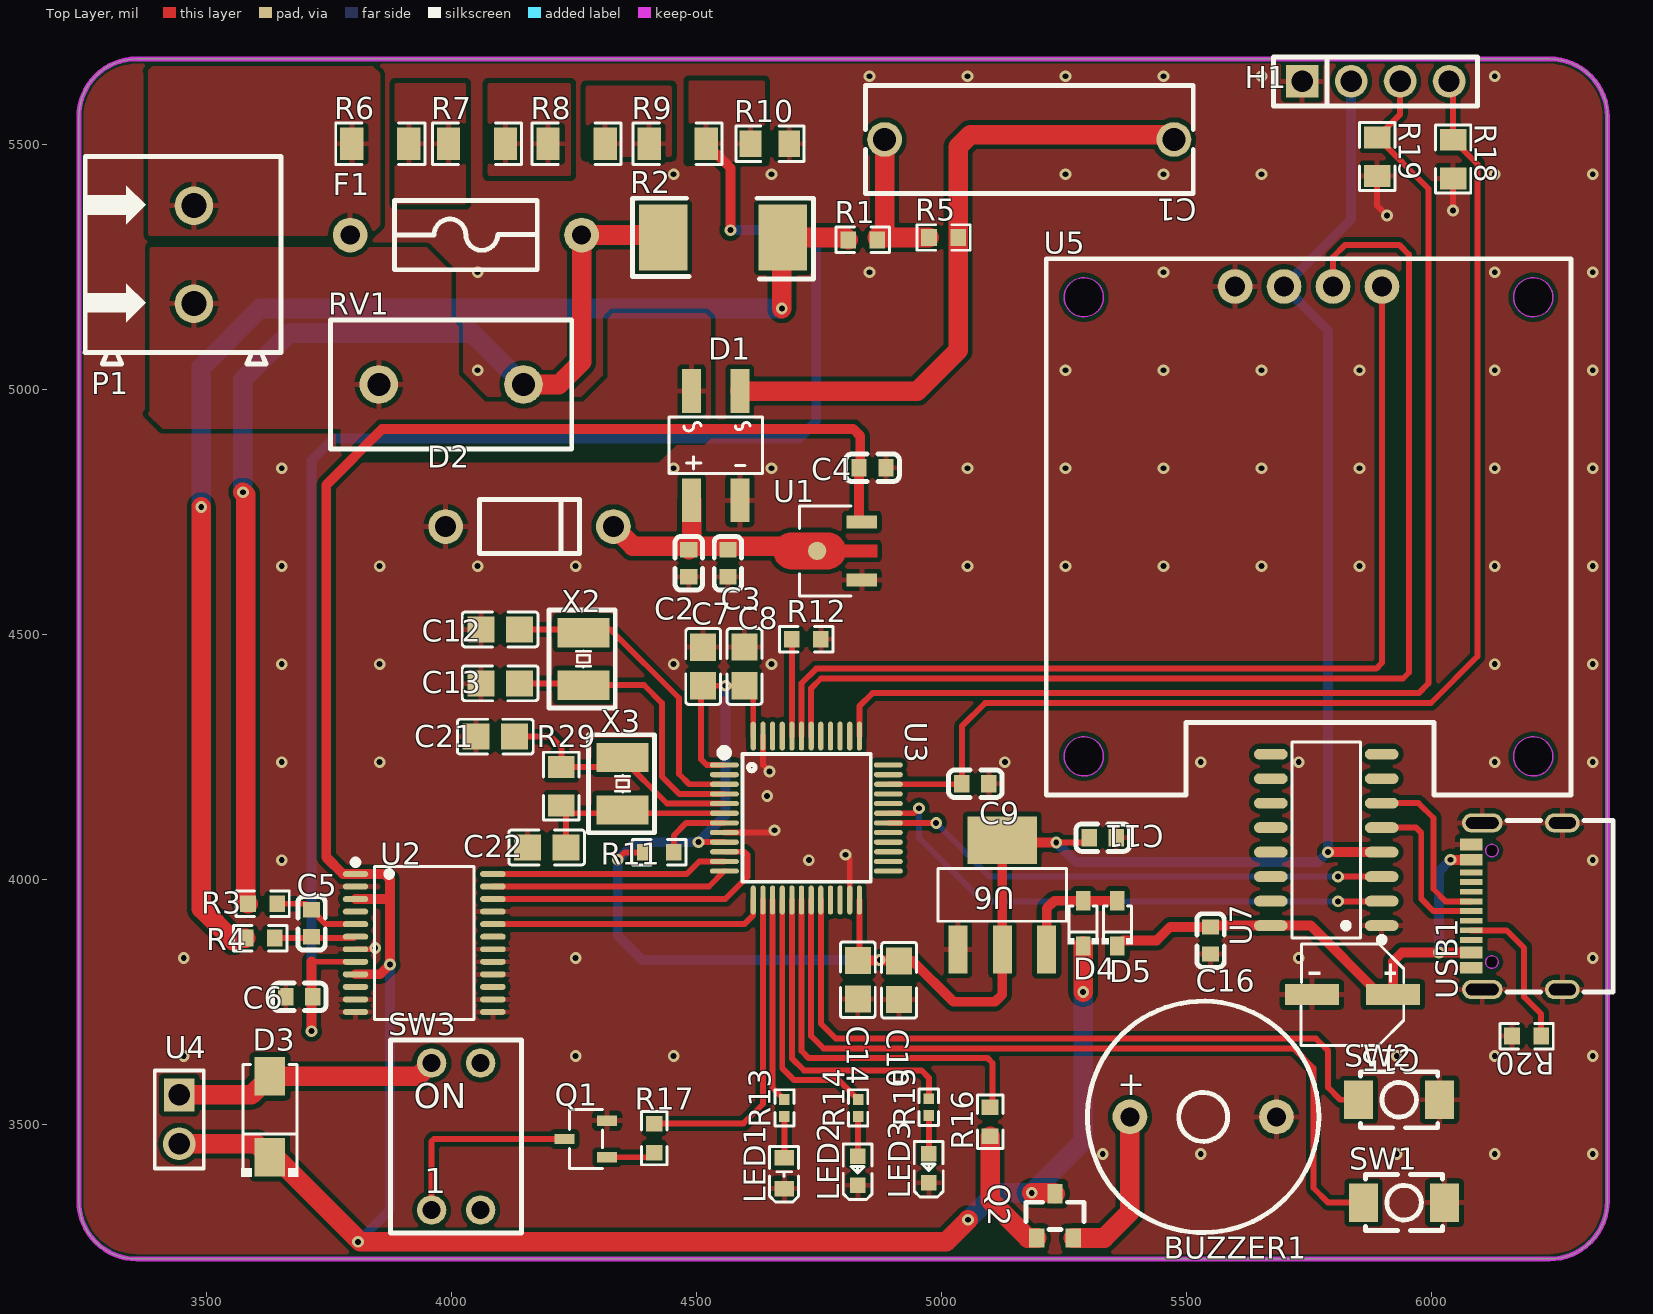
[diagram p0: Top Layer view]
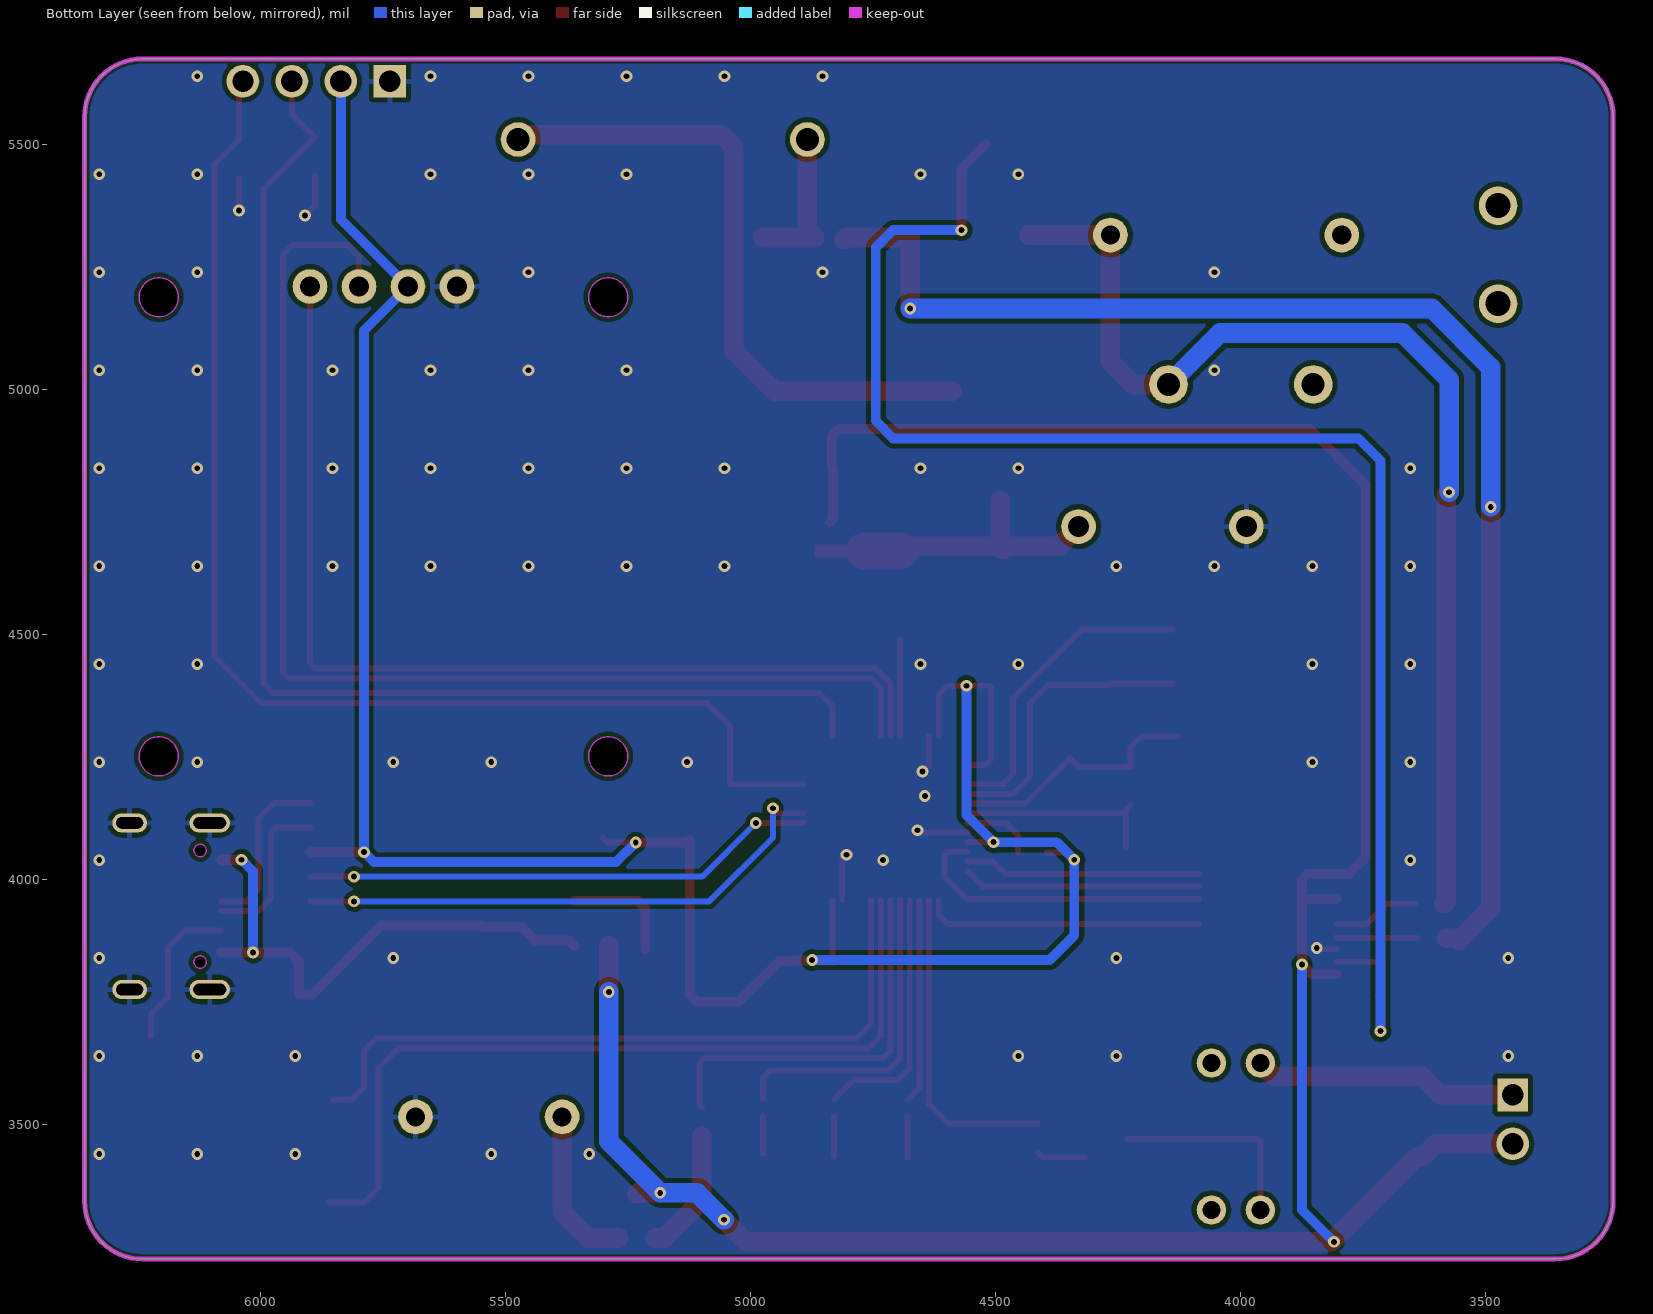
[diagram p1: Bottom Layer view, seen from below]
# Altium PCB MISC49877.pcbdoc
Units mil, origin at the board's own origin, x right, y up, seen from the top; angles counter-clockwise.
Board outline 3120 x 2449.61 mil, 2 copper layers (Top Layer, Bottom Layer), stack 2.757 mil thick; 67 components, 52 nets, 243 pads, 106 vias.

## Layer stack, top to bottom
Top Solder Mask Layer: solder mask 0.394, Dk 3.3
Top Layer: signal copper 1.379
Bottom Layer: signal copper 1.378
Bottom Solder Mask Layer: solder mask 0.394, Dk 3.3

## Board outline
3358.11,5674.61 ccw(c3358.11,5556.5) 3240,5556.5 3240,3343.11 ccw(c3358.11,3343.11) 3358.11,3225 6241.89,3225 ccw(c6241.89,3343.11) 6360,3343.11 6360,5556.5 ccw(c6241.89,5556.5) 6241.89,5674.61 3358.11,5674.61

## Design rules (kind name [scope] priority, off if disabled: settings)
BoardOutlineClearance Plane_innerPlane_1 [All] p2 off: genericclearance=4 ignorepadtopadclearanceinfootprint=FALSE except(0: Arc-SplitContinuation Track-SplitContinuation SMDPad-SplitContinuation THPad-SplitContinuation Via-SplitContinuation Fill-SplitContinuation Region-SplitContinuation Poly-SplitContinuation Text-SplitContinuation Hole-SplitContinuation; 6: Arc-CutoutEdge Track-CutoutEdge SMDPad-CutoutEdge THPad-CutoutEdge Via-CutoutEdge Text-CutoutEdge; 6.9: Hole-OutlineEdge Hole-CutoutEdge; 10: Poly-OutlineEdge Poly-CutoutEdge; 11.8: Arc-OutlineEdge Track-OutlineEdge SMDPad-OutlineEdge THPad-OutlineEdge Via-OutlineEdge Fill-OutlineEdge Region-OutlineEdge Text-OutlineEdge Fill-CutoutEdge Region-CutoutEdge)
BoardOutlineClearance Copper_copperRegion_1 [All] p4 off: genericclearance=4 ignorepadtopadclearanceinfootprint=FALSE except(0: Arc-SplitContinuation Track-SplitContinuation SMDPad-SplitContinuation THPad-SplitContinuation Via-SplitContinuation Fill-SplitContinuation Region-SplitContinuation Poly-SplitContinuation Text-SplitContinuation Hole-SplitContinuation; 6: Arc-CutoutEdge Track-CutoutEdge SMDPad-CutoutEdge THPad-CutoutEdge Via-CutoutEdge Text-CutoutEdge; 6.9: Hole-OutlineEdge Hole-CutoutEdge; 10: Poly-OutlineEdge Poly-CutoutEdge; 11.8: Arc-OutlineEdge Track-OutlineEdge SMDPad-OutlineEdge THPad-OutlineEdge Via-OutlineEdge Fill-OutlineEdge Region-OutlineEdge Text-OutlineEdge Fill-CutoutEdge Region-CutoutEdge)
BoardOutlineClearance Copper_copperRegion_copperThickness1oz_1 [All] p6 off: genericclearance=4 ignorepadtopadclearanceinfootprint=FALSE except(0: Arc-SplitContinuation Track-SplitContinuation SMDPad-SplitContinuation THPad-SplitContinuation Via-SplitContinuation Fill-SplitContinuation Region-SplitContinuation Poly-SplitContinuation Text-SplitContinuation Hole-SplitContinuation; 6: Arc-CutoutEdge Track-CutoutEdge SMDPad-CutoutEdge THPad-CutoutEdge Via-CutoutEdge Text-CutoutEdge; 6.9: Hole-OutlineEdge Hole-CutoutEdge; 10: Poly-OutlineEdge Poly-CutoutEdge; 11.8: Arc-OutlineEdge Track-OutlineEdge SMDPad-OutlineEdge THPad-OutlineEdge Via-OutlineEdge Fill-OutlineEdge Region-OutlineEdge Text-OutlineEdge Fill-CutoutEdge Region-CutoutEdge)
BoardOutlineClearance Copper_copperRegion_Copper_copperRegion_1 [All] p8 off: genericclearance=4 ignorepadtopadclearanceinfootprint=FALSE except(0: Arc-SplitContinuation Track-SplitContinuation SMDPad-SplitContinuation THPad-SplitContinuation Via-SplitContinuation Fill-SplitContinuation Region-SplitContinuation Poly-SplitContinuation Text-SplitContinuation Hole-SplitContinuation; 6: Arc-CutoutEdge Track-CutoutEdge SMDPad-CutoutEdge THPad-CutoutEdge Via-CutoutEdge Text-CutoutEdge; 6.9: Hole-OutlineEdge Hole-CutoutEdge; 10: Poly-OutlineEdge Poly-CutoutEdge; 11.8: Arc-OutlineEdge Track-OutlineEdge SMDPad-OutlineEdge THPad-OutlineEdge Via-OutlineEdge Fill-OutlineEdge Region-OutlineEdge Text-OutlineEdge Fill-CutoutEdge Region-CutoutEdge)
BoardOutlineClearance copperThickness1oz_1 [All] p10: genericclearance=4 ignorepadtopadclearanceinfootprint=FALSE except(0: Arc-SplitContinuation Track-SplitContinuation SMDPad-SplitContinuation THPad-SplitContinuation Via-SplitContinuation Fill-SplitContinuation Region-SplitContinuation Poly-SplitContinuation Text-SplitContinuation Hole-SplitContinuation; 6: Arc-CutoutEdge Track-CutoutEdge SMDPad-CutoutEdge THPad-CutoutEdge Via-CutoutEdge Text-CutoutEdge; 6.9: Hole-OutlineEdge Hole-CutoutEdge; 10: Poly-OutlineEdge Poly-CutoutEdge; 11.8: Arc-OutlineEdge Track-OutlineEdge SMDPad-OutlineEdge THPad-OutlineEdge Via-OutlineEdge Fill-OutlineEdge Region-OutlineEdge Text-OutlineEdge Fill-CutoutEdge Region-CutoutEdge)
Clearance Plane_innerPlane [All] p1 off: gap=4 ignorepadtopadclearanceinfootprint=FALSE except(6: SMDPad-Track SMDPad-SMDPad THPad-Track SMDPad-THPad THPad-THPad Track-Via SMDPad-Via THPad-Via Via-Via Fill-SMDPad Region-SMDPad Fill-THPad Region-THPad Fill-Via Region-Via Fill-Fill Fill-Region Region-Region Arc-Track Arc-SMDPad Arc-THPad Arc-Via Fill-Arc Region-Arc Arc-Arc Text-Track SMDPad-Text Text-THPad Text-Via Fill-Text Region-Text Arc-Text Text-Text; 6.9: Hole-Track Hole-SMDPad Hole-THPad Hole-Via Fill-Hole Region-Hole Hole-Arc Hole-Text; 10: Poly-Track Poly-SMDPad Poly-THPad Poly-Via Poly-Fill Poly-Region Poly-Poly Poly-Arc Poly-Text Poly-Hole; 11.8: Fill-Track Region-Track)
Clearance Copper_copperRegion [All] p3 off: gap=4 ignorepadtopadclearanceinfootprint=FALSE except(6: SMDPad-Track SMDPad-SMDPad THPad-Track SMDPad-THPad THPad-THPad Track-Via SMDPad-Via THPad-Via Via-Via Fill-SMDPad Region-SMDPad Fill-THPad Region-THPad Fill-Via Region-Via Fill-Fill Fill-Region Region-Region Arc-Track Arc-SMDPad Arc-THPad Arc-Via Fill-Arc Region-Arc Arc-Arc Text-Track SMDPad-Text Text-THPad Text-Via Fill-Text Region-Text Arc-Text Text-Text; 6.9: Hole-Track Hole-SMDPad Hole-THPad Hole-Via Fill-Hole Region-Hole Hole-Arc Hole-Text; 10: Poly-Track Poly-SMDPad Poly-THPad Poly-Via Poly-Fill Poly-Region Poly-Poly Poly-Arc Poly-Text Poly-Hole; 11.8: Fill-Track Region-Track)
Clearance Copper_copperRegion_copperThickness1oz [All] p5 off: gap=4 ignorepadtopadclearanceinfootprint=FALSE except(6: SMDPad-Track SMDPad-SMDPad THPad-Track SMDPad-THPad THPad-THPad Track-Via SMDPad-Via THPad-Via Via-Via Fill-SMDPad Region-SMDPad Fill-THPad Region-THPad Fill-Via Region-Via Fill-Fill Fill-Region Region-Region Arc-Track Arc-SMDPad Arc-THPad Arc-Via Fill-Arc Region-Arc Arc-Arc Text-Track SMDPad-Text Text-THPad Text-Via Fill-Text Region-Text Arc-Text Text-Text; 6.9: Hole-Track Hole-SMDPad Hole-THPad Hole-Via Fill-Hole Region-Hole Hole-Arc Hole-Text; 10: Poly-Track Poly-SMDPad Poly-THPad Poly-Via Poly-Fill Poly-Region Poly-Poly Poly-Arc Poly-Text Poly-Hole; 11.8: Fill-Track Region-Track)
Clearance Copper_copperRegion_Copper_copperRegion [All] p7 off: gap=4 ignorepadtopadclearanceinfootprint=FALSE except(6: SMDPad-Track SMDPad-SMDPad THPad-Track SMDPad-THPad THPad-THPad Track-Via SMDPad-Via THPad-Via Via-Via Fill-SMDPad Region-SMDPad Fill-THPad Region-THPad Fill-Via Region-Via Fill-Fill Fill-Region Region-Region Arc-Track Arc-SMDPad Arc-THPad Arc-Via Fill-Arc Region-Arc Arc-Arc Text-Track SMDPad-Text Text-THPad Text-Via Fill-Text Region-Text Arc-Text Text-Text; 6.9: Hole-Track Hole-SMDPad Hole-THPad Hole-Via Fill-Hole Region-Hole Hole-Arc Hole-Text; 10: Poly-Track Poly-SMDPad Poly-THPad Poly-Via Poly-Fill Poly-Region Poly-Poly Poly-Arc Poly-Text Poly-Hole; 11.8: Fill-Track Region-Track)
Clearance copperThickness1oz [All] p9: gap=4 ignorepadtopadclearanceinfootprint=FALSE except(6: SMDPad-Track SMDPad-SMDPad THPad-Track SMDPad-THPad THPad-THPad Track-Via SMDPad-Via THPad-Via Via-Via Fill-SMDPad Region-SMDPad Fill-THPad Region-THPad Fill-Via Region-Via Fill-Fill Fill-Region Region-Region Arc-Track Arc-SMDPad Arc-THPad Arc-Via Fill-Arc Region-Arc Arc-Arc Text-Track SMDPad-Text Text-THPad Text-Via Fill-Text Region-Text Arc-Text Text-Text; 6.9: Hole-Track Hole-SMDPad Hole-THPad Hole-Via Fill-Hole Region-Hole Hole-Arc Hole-Text; 10: Poly-Track Poly-SMDPad Poly-THPad Poly-Via Poly-Fill Poly-Region Poly-Poly Poly-Arc Poly-Text Poly-Hole; 11.8: Fill-Track Region-Track)
DiffPairsRouting differentialPair [All] p1: maxlimit=6 minlimit=5 mostfreqgap=6 toplayer_minwidth=5 toplayer_prefwidth=100 toplayer_maxwidth=100 toplayer_mingap=5 toplayer_prefgap=6 toplayer_maxgap=6 bottomlayer_minwidth=5 bottomlayer_prefwidth=100 bottomlayer_maxwidth=100 bottomlayer_mingap=5 bottomlayer_prefgap=6 bottomlayer_maxgap=6 maxuncoupledlength=10
HoleToHoleClearance otherClearance [All] p1: gap=11.8 allowstackedmicrovias=TRUE
Length netLength [All] p1: minlimit=0 maxlimit=0
MatchedLengths netLengthTolerance [All] p1: tolerance=1000
PasteMaskExpansion pasteMaskExpansion [All] p1: expansion=0
PlaneConnect innerPlane [All] p1: planeconnectstyle=Relief reliefexpansion=20 reliefentries=4 reliefconductorwidth=10 reliefairgap=10
PolygonConnect copperRegion_copperThickness1oz [All] p1 off: connectstyle=Relief reliefconductorwidth=10 reliefentries=4 polygonreliefangle="90 Angle" airgapwidth=10 via.connectstyle=Relief via.reliefconductorwidth=10 via.reliefentries=4 via.polygonreliefangle="90 Angle" via.airgapwidth=10
PolygonConnect copperRegion_Copper_copperRegion [All] p2 off: connectstyle=Relief reliefconductorwidth=10 reliefentries=4 polygonreliefangle="90 Angle" airgapwidth=10 via.connectstyle=Relief via.reliefconductorwidth=10 via.reliefentries=4 via.polygonreliefangle="90 Angle" via.airgapwidth=10
PolygonConnect copperRegion [All] p3: connectstyle=Direct reliefconductorwidth=10 reliefentries=4 polygonreliefangle="90 Angle" airgapwidth=10 via.connectstyle=Relief via.reliefconductorwidth=10 via.reliefentries=4 via.polygonreliefangle="90 Angle" via.airgapwidth=10
RoutingVias viaSize [All] p1: holewidth=12 width=24 viastyle="Through Hole" minholewidth=1 minwidth=1 maxholewidth=393.7 maxwidth=248
SolderMaskExpansion solderMaskExpansion [IsVia] p1: expansion=-1000 istentingtop=TRUE
SolderMaskExpansion solderMaskExpansion [All] p2: expansion=2 istentingtop=FALSE
Width copperThickness1oz_2 [All] p1: maxlimit=100 minlimit=5 preferedwidth=10

## Components (designator, comment, footprint, x,y, rotation, side; value= is the part's Value field where it differs from the comment)
BUZZER1 "2.4kHz" BUZ-TH_BD12.0-P7.60-D0.6-FD 5535,3515 r0 top
C1 "470nF" CAP-TH_L17.0-W5.5-P15.00-D1.2 5180,5510 r180 top
C2 "100μF" C0603 4485,4645 r90 top
C3 "0.1μF" C0603 4565,4645 r270 top
C4 "10μF" C0603 4860,4840 r180 top
C5 "1nF" C0603 3715,3910 r90 top
C6 "1nF" C0603 3690,3760 r0 top
C7 "100nF" C0805 4514.37,4434.37 r90 top
C8 "100nF" C0805 4598.8,4434.51 r270 top
C9 "100nF" C0603 5070,4195 r180 top
C10 "100nF" C0805 4914.37,3793.97 r270 top
C11 "100nF" C0603 5330,4085 r180 top
C12 "20pF" C0805 4100,4510 r180 top
C13 "20pF" C0805 4100,4400 r0 top
C14 "100nF" C0805 4830,3795 r90 top
C15 "10uF" CAP-SMD_BD5.0-L5.3-W5.3-FD 5839.64,3765 r180 top
C16 "100nF" C0603 5550,3875 r90 top
C21 "20pF" C0805 4090.21,4291.12 r0 top
C22 "20pF" C0805 4195,4065 r0 top
D1 "MB10S" MBS_L4.7-W4.0-P2.50-LS7.0-TL 4540,4885 r270 top
D2 "1N4742" DO-41_BD2.4-L4.7-P8.70-D0.8-FD 4160,4720 r0 top
D3 "1N4007" SMA_L4.3-W2.5-LS5.0-RD 3630,3515 r90 top
D4 "1N5819WS" SOD-323_L1.8-W1.3-LS2.5-RD 5290,3910 r90 top
D5 "1N5819WS" SOD-323_L1.8-W1.3-LS2.5-RD 5360,3910 r90 top
F1 "2F.0500212000S1B02" FUSE-TH_BD3.0-L7.2-P11.20-D0.6 4030,5315 r0 top
H1 "" HDR-TH_4P-P2.54-V-F 5887,5628.78 r0 top
LED1 "NCD0603G1" LED0603-RD_1 4679.87,3400.05 r90 top
LED2 "NCD0603R1" LED0603-RD_RED 4830,3405 r90 top
LED3 "NCD0603Y1" LED0603-RD 4975,3410 r90 top
P1 "WJ500V-5.08-2P" CONN-TH_2P-P5.00_WJ500V-5.08-2P 3475,5275 r90 top
Q1 "S8050 J3Y(RANGE:200-350)" SOT-23-3_L3.0-W1.7-P0.95-LS2.9-BR 4275,3470 r0 top
Q2 "" S8050_SOT-23 5232.54,3313.14 r270 top
R1 "10Ω" R0603 4840,5305 r0 top
R2 "2mΩ" RES-SMD_L6.4-W3.2-1 4555,5310 r0 top
R3 "1K" R0603 3615,3950 r0 top
R4 "1K" R0603 3610,3880 r0 top
R5 "1MΩ" R0603 5005,5310 r0 top
R6 "1MΩ" R1206 3855.45,5501.36 r0 top
R7 "1MΩ" R1206 4052.86,5501.36 r0 top
R8 "1MΩ" R1206 4256.06,5501.36 r0 top
R9 "1MΩ" R1206 4462.27,5501.36 r0 top
R10 "10kΩ" R0805 4650.66,5501.36 r0 top
R11 "10K" R0603 4425,4055 r0 top
R12 "10K" R0603 4725,4490 r0 top
R13 "220Ω" R0402 4680.3,3533.26 r90 top
R14 "220Ω" R0402 4830.69,3533.26 r90 top
R15 "220Ω" R0402 4975,3535 r90 top
R16 "1KΩ" R0603 5100,3505 r90 top
R17 "1KΩ" R0603 4414.48,3471.81 r270 top
R18 "10kΩ" R0805 6045,5470 r270 top
R19 "10kΩ" R0805 5890,5475 r270 top
R20 "5.1K" R0603 6195,3680 r180 top
R29 "1M" R0805 4225,4190 r90 top
RV1 "190pF@1kHz" RES-TH_L12.5-W6.7-P7.50-D1.2 4000,5010 r0 top
SW1 "TS3425A2P 250gf" SW-SMD_L3.9-W2.9-LS5.0 5945,3340 r0 top
SW2 "TS3425A2P 250gf" SW-SMD_L3.9-W2.9-LS5.0 5935,3550 r0 top
SW3 "BSE02GR" SW-TH_4P-L9.9-W6.8-P7.62-BL 4010,3475 r0 top
U1 "HT7550-1" SOT-89_L4.5-W2.5-P1.50-LS4.2-BR 4785,4670 r0 top
U2 "ADE7755ARSZ" SSOP-24_L8.1-W5.3-P0.65-LS7.8-BL 3945,3870 r270 top
U3 "STM32F030C8T6TR" LQFP-48_L7.0-W7.0-P0.50-LS9.0-BL 4725,4125 r270 top
U4 "KF301-5.0-2P" HDR-M-2.54_1X2 3445,3510 r270 top
U5 "HS96L03W2C03" OLED-TH_L27.8-W27.2-P2.54_C9900033791 5750,5210 r0 top
U6 "AMS1117-3.3" SOT-223-4_L6.5-W3.5-P2.30-LS7.0-BR 5125,3968.34 r270 top
U7 "CH340C" SOP-16_L10.0-W3.9-P1.27-LS6.0-BL 5786.23,4080.41 r90 top
USB1 "TYPE-C16PIN" USB-C-SMD_TYPE-C16PIN 6175,3945 r90 top
X2 "32.768MHz" CRYSTAL-SMD_L3.2-W2.5_3225-8MHZ 4270,4450 r90 top
X3 "8MHz" CRYSTAL-SMD_L3.2-W2.5_3225-8MHZ 4350,4195 r90 top

## Footprints (in the part's own frame and the unit in brackets; to place one, negate y for a bottom-side part, rotate by r counter-clockwise, add the part's x,y. Pads: shape width x height; smd on the part's side, far side on the other; paste and mask are expansions set on the pad)
BUZ-TH_BD12.0-P7.60-D0.6-FD [mm]
  round 1.8 hole 1: 1(-3.8,0) 2(3.8,0)
  silkscreen extent -6,-6 6,6
C0603 [mm]
  rect 0.8x0.9 smd: 1(-0.7,0) 2(0.7,0)
  silkscreen extent -1.39,-0.71 1.39,0.71
C0805 [mm]
  rect 1.41x1.35 smd paste-100 mask+0.051: 1(-1,0) 2(1,0)
  silkscreen extent -1.96,-0.9 1.96,0.9
CAP-SMD_BD5.0-L5.3-W5.3-FD [mm]
  rect 2.8x1.1 smd: 1(-2.1,0) 2(2.1,0)
  silkscreen extent -2.66,-2.62 2.66,2.65
CAP-TH_L17.0-W5.5-P15.00-D1.2 [mm]
  round 1.8 hole 1.2: 1(-7.501,0) 2(7.501,0)
  silkscreen extent -8.5,-2.8 8.5,2.8
CONN-TH_2P-P5.00_WJ500V-5.08-2P [mm]
  round 2 hole 1.3: 1(-2.54,0) 2(2.54,0)
  silkscreen extent -5.68,-4.52 5.08,5.64
CRYSTAL-SMD_L3.2-W2.5_3225-8MHZ [mil]
  rect 60x106.3 smd paste+0 mask+1.97: 1(-53.62,0) 2(53.62,0)
  silkscreen extent -100,-65 100,70
DO-41_BD2.4-L4.7-P8.70-D0.8-FD [mm]
  round 1.8 hole 1.1: 1(-4.35,0) 2(4.35,0)
  silkscreen extent -2.6,-1.4 2.6,1.4
FUSE-TH_BD3.0-L7.2-P11.20-D0.6 [mm]
  round 1.8 hole 1: 1(-6,0) 2(6,0)
  silkscreen extent -3.7,-1.8 3.7,1.8
HDR-M-2.54_1X2 [mm]
  rect 1.7x1.575 hole 1.1: 1(-1.27,0)
  round 1.7 hole 1.1: 2(1.27,0)
  silkscreen extent -2.54,-1.27 2.54,1.27
HDR-TH_4P-P2.54-V-F [mm]
  rect 1.7x1.7 hole 1.1: 1(-3.81,0)
  round 1.7 hole 1.1: 2(-1.27,0) 3(1.27,0) 4(3.81,0)
  silkscreen extent -5.29,-1.27 5.29,1.27
LED0603-RD [mm]
  rect 0.8x0.8 smd: 1(-0.749,0) 2(0.749,0)
  silkscreen extent -1.49,-0.75 1.39,0.76
LED0603-RD_1 [mm]
  rect 0.8x1 smd: 1(-0.799,-0.004) 2(0.799,0.004)
  silkscreen extent -1.49,-0.75 1.39,0.76
LED0603-RD_RED [mm]
  rect 0.8x0.8 smd: 1(-0.749,-0.003) 2(0.749,0.003)
  silkscreen extent -1.49,-0.75 1.39,0.76
LQFP-48_L7.0-W7.0-P0.50-LS9.0-BL [mm]
  oval 0.27x1.5 smd paste+0 mask+0.05: 1(-2.75,-4.25) 2(-2.25,-4.25) 3(-1.75,-4.25) 4(-1.25,-4.25) 5(-0.75,-4.25) 6(-0.25,-4.25) 7(0.25,-4.25) 8(0.75,-4.25) 9(1.25,-4.25) 10(1.75,-4.25) 11(2.25,-4.25) 12(2.75,-4.25) 25(2.75,4.25) 26(2.25,4.25) 27(1.75,4.25) 28(1.25,4.25) 29(0.75,4.25) 30(0.25,4.25) 31(-0.25,4.25) 32(-0.75,4.25) 33(-1.25,4.25) 34(-1.75,4.25) 35(-2.25,4.25) 36(-2.75,4.25)
  oval 1.5x0.27 smd paste+0 mask+0.05: 13(4.25,-2.75) 14(4.25,-2.25) 15(4.25,-1.75) 16(4.25,-1.25) 17(4.25,-0.75) 18(4.25,-0.25) 19(4.25,0.25) 20(4.25,0.75) 21(4.25,1.25) 22(4.25,1.75) 23(4.25,2.25) 24(4.25,2.75) 37(-4.25,2.75) 38(-4.25,2.25) 39(-4.25,1.75) 40(-4.25,1.25) 41(-4.25,0.75) 42(-4.25,0.25) 43(-4.25,-0.25) 44(-4.25,-0.75) 45(-4.25,-1.25) 46(-4.25,-1.75) 47(-4.25,-2.25) 48(-4.25,-2.75)
  silkscreen extent -3.59,-4.46 3.3,3.34
MBS_L4.7-W4.0-P2.50-LS7.0-TL [mm]
  rect 2.265x0.98 smd: 1(-2.832,1.25) 2(-2.832,-1.25) 3(2.832,-1.25) 4(2.832,1.25)
  silkscreen extent -1.5,-2.43 1.44,2.43
OLED-TH_L27.8-W27.2-P2.54_C9900033791 [mm]
  round 1.8 hole 1.05 paste+0 mask+0.05: 1(-3.81,0) 2(-1.27,0) 3(1.27,0) 4(3.81,0)
  Board Outline Layer circle w0.003: c-11.65,-0.56 r1.016
  Board Outline Layer circle w0.003: c11.65,-0.56 r1.016
  Board Outline Layer circle w0.003: c-11.65,-24.36 r1.016
  Board Outline Layer circle w0.003: c11.65,-24.36 r1.016
  Board Outline Layer region: -10.634,-0.56 -10.735,-1.001 -11.016,-1.354 -11.424,-1.551 -11.876,-1.551 -12.283,-1.354 -12.565,-1.001 -12.666,-0.56 -12.666,-0.56 -12.565,-0.119 -12.283,0.234 -11.876,0.431 -11.424,0.431 -11.016,0.234 -10.735,-0.119 -10.634,-0.56
  Board Outline Layer region: -10.634,-0.56 -10.643,-0.698 -10.672,-0.834 -10.718,-0.965 -10.782,-1.088 -10.862,-1.201 -10.956,-1.303 -11.064,-1.39 -11.183,-1.462 -11.31,-1.517 -11.443,-1.555 -11.581,-1.574 -11.719,-1.574 -11.857,-1.555 -11.99,-1.517 -12.117,-1.462 -12.236,-1.39 -12.343,-1.303 -12.438,-1.201 -12.518,-1.088 -12.582,-0.965 -12.628,-0.834 -12.656,-0.698 -12.666,-0.56 -12.656,-0.422 -12.628,-0.286 -12.582,-0.155 -12.518,-0.032 -12.438,0.081 -12.343,0.183 -12.236,0.27 -12.117,0.342 -11.99,0.397 -11.857,0.435 -11.719,0.454 -11.581,0.454 -11.443,0.435 -11.31,0.397 -11.183,0.342 -11.064,0.27 -10.956,0.183 -10.862,0.081 -10.782,-0.032 -10.718,-0.155 -10.672,-0.286 -10.643,-0.422
  Board Outline Layer region: 12.666,-0.56 12.565,-1.001 12.283,-1.354 11.876,-1.551 11.424,-1.551 11.017,-1.354 10.735,-1.001 10.634,-0.56 10.634,-0.56 10.735,-0.119 11.017,0.234 11.424,0.431 11.876,0.431 12.283,0.234 12.565,-0.119 12.666,-0.56
  Board Outline Layer region: 12.666,-0.56 12.657,-0.698 12.628,-0.834 12.582,-0.965 12.518,-1.088 12.438,-1.201 12.343,-1.303 12.236,-1.39 12.117,-1.462 11.99,-1.517 11.857,-1.555 11.719,-1.574 11.581,-1.574 11.443,-1.555 11.31,-1.517 11.183,-1.462 11.064,-1.39 10.957,-1.303 10.862,-1.201 10.782,-1.088 10.718,-0.965 10.672,-0.834 10.643,-0.698 10.634,-0.56 10.643,-0.422 10.672,-0.286 10.718,-0.155 10.782,-0.032 10.862,0.081 10.957,0.183 11.064,0.27 11.183,0.342 11.31,0.397 11.443,0.435 11.581,0.454 11.719,0.454 11.857,0.435 11.99,0.397 12.117,0.342 12.236,0.27 12.343,0.183 12.438,0.081 12.518,-0.032 12.582,-0.155 12.628,-0.286 12.657,-0.422
  Board Outline Layer region: -10.634,-24.36 -10.735,-24.801 -11.016,-25.154 -11.424,-25.35 -11.876,-25.35 -12.283,-25.154 -12.565,-24.801 -12.666,-24.36 -12.666,-24.36 -12.565,-23.919 -12.283,-23.566 -11.876,-23.369 -11.424,-23.369 -11.016,-23.566 -10.735,-23.919 -10.634,-24.36
  Board Outline Layer region: -10.634,-24.36 -10.643,-24.498 -10.672,-24.634 -10.718,-24.765 -10.782,-24.888 -10.862,-25.001 -10.956,-25.102 -11.064,-25.19 -11.183,-25.262 -11.31,-25.317 -11.443,-25.355 -11.581,-25.374 -11.719,-25.374 -11.857,-25.355 -11.99,-25.317 -12.117,-25.262 -12.236,-25.19 -12.343,-25.102 -12.438,-25.001 -12.518,-24.888 -12.582,-24.765 -12.628,-24.634 -12.656,-24.498 -12.666,-24.36 -12.656,-24.222 -12.628,-24.086 -12.582,-23.955 -12.518,-23.832 -12.438,-23.719 -12.343,-23.617 -12.236,-23.53 -12.117,-23.458 -11.99,-23.403 -11.857,-23.365 -11.719,-23.346 -11.581,-23.346 -11.443,-23.365 -11.31,-23.403 -11.183,-23.458 -11.064,-23.53 -10.956,-23.617 -10.862,-23.719 -10.782,-23.832 -10.718,-23.955 -10.672,-24.086 -10.643,-24.222
  Board Outline Layer region: 12.666,-24.36 12.565,-24.801 12.283,-25.154 11.876,-25.35 11.424,-25.35 11.017,-25.154 10.735,-24.801 10.634,-24.36 10.634,-24.36 10.735,-23.919 11.017,-23.566 11.424,-23.369 11.876,-23.369 12.283,-23.566 12.565,-23.919 12.666,-24.36
  Board Outline Layer region: 12.666,-24.36 12.657,-24.498 12.628,-24.634 12.582,-24.765 12.518,-24.888 12.438,-25.001 12.343,-25.102 12.236,-25.19 12.117,-25.262 11.99,-25.317 11.857,-25.355 11.719,-25.374 11.581,-25.374 11.443,-25.355 11.31,-25.317 11.183,-25.262 11.064,-25.19 10.957,-25.102 10.862,-25.001 10.782,-24.888 10.718,-24.765 10.672,-24.634 10.643,-24.498 10.634,-24.36 10.643,-24.222 10.672,-24.086 10.718,-23.955 10.782,-23.832 10.862,-23.719 10.957,-23.617 11.064,-23.53 11.183,-23.458 11.31,-23.403 11.443,-23.365 11.581,-23.346 11.719,-23.346 11.857,-23.365 11.99,-23.403 12.117,-23.458 12.236,-23.53 12.343,-23.617 12.438,-23.719 12.518,-23.832 12.582,-23.955 12.628,-24.086 12.657,-24.222
  Multi-Layer board cut-out: -10.634,-0.56 -10.735,-1.001 -11.016,-1.354 -11.424,-1.551 -11.876,-1.551 -12.283,-1.354 -12.565,-1.001 -12.666,-0.56 -12.666,-0.56 -12.565,-0.119 -12.283,0.234 -11.876,0.431 -11.424,0.431 -11.016,0.234 -10.735,-0.119 -10.634,-0.56
  Multi-Layer board cut-out: 12.666,-0.56 12.565,-1.001 12.283,-1.354 11.876,-1.551 11.424,-1.551 11.017,-1.354 10.735,-1.001 10.634,-0.56 10.634,-0.56 10.735,-0.119 11.017,0.234 11.424,0.431 11.876,0.431 12.283,0.234 12.565,-0.119 12.666,-0.56
  Multi-Layer board cut-out: -10.634,-24.36 -10.735,-24.801 -11.016,-25.154 -11.424,-25.35 -11.876,-25.35 -12.283,-25.154 -12.565,-24.801 -12.666,-24.36 -12.666,-24.36 -12.565,-23.919 -12.283,-23.566 -11.876,-23.369 -11.424,-23.369 -11.016,-23.566 -10.735,-23.919 -10.634,-24.36
  Multi-Layer board cut-out: 12.666,-24.36 12.565,-24.801 12.283,-25.154 11.876,-25.35 11.424,-25.35 11.017,-25.154 10.735,-24.801 10.634,-24.36 10.634,-24.36 10.735,-23.919 11.017,-23.566 11.424,-23.369 11.876,-23.369 12.283,-23.566 12.565,-23.919 12.666,-24.36
  silkscreen extent -13.6,-26.36 13.6,1.44
R0402 [mm]
  rect 0.566x0.54 smd paste-100 mask+0.051: 1(-0.433,0) 2(0.433,0)
  silkscreen extent -0.94,-0.5 0.94,0.5
R0603 [mil]
  rect 31.75x34.02 smd paste-3937.01 mask+2: 1(-29.66,0) 2(29.66,0)
  silkscreen extent -55,-26 55,26
R0805 [mm]
  rect 1.133x1.377 smd paste-100 mask+0.051: 1(-1,0) 2(1,0)
  silkscreen extent -1.76,-0.92 1.76,0.92
R1206 [mil]
  rect 47.54x66.97 smd paste-3937.01 mask+2: 1(-58.22,0) 2(58.22,0)
  silkscreen extent -91,-42 91,42
RES-SMD_L6.4-W3.2-1 [mm]
  rect 2.5x3.4 smd: 1(-3.1,0) 2(3.1,0)
  silkscreen extent -4.69,-2.16 4.69,2.03
RES-TH_L12.5-W6.7-P7.50-D1.2 [mm]
  round 2 hole 1.2: 1(-3.749,0) 2(3.749,0)
  silkscreen extent -6.25,-3.35 6.25,3.35
S8050_SOT-23 [mm]
  rect 1x0.8 smd paste+0 mask+0.051: 1(1.15,-0.95) 2(1.15,0.95) 3(-1.15,0)
  silkscreen extent -0.7,-1.5 0.7,1.5
SMA_L4.3-W2.5-LS5.0-RD [mm]
  rect 2x1.593 smd: 1(-2.1,0) 2(2.1,0)
  silkscreen extent -3.11,-1.48 2.73,1.48
SOD-323_L1.8-W1.3-LS2.5-RD [mm]
  rect 1x0.75 smd: 1(-1.173,0) 2(1.173,0)
  silkscreen extent -1.08,-0.8 0.9,0.8
SOP-16_L10.0-W3.9-P1.27-LS6.0-BL [mm]
  oval 0.56x1.745 smd: 1(-4.445,-2.872) 2(-3.175,-2.872) 3(-1.905,-2.872) 4(-0.635,-2.872) 5(0.635,-2.872) 6(1.905,-2.872) 7(3.175,-2.872) 8(4.445,-2.872) 9(4.445,2.872) 10(3.175,2.872) 11(1.905,2.872) 12(0.635,2.872) 13(-0.635,2.872) 14(-1.905,2.872) 15(-3.175,2.872) 16(-4.445,2.872)
  silkscreen extent -5.33,-3.02 5.08,1.77
SOT-23-3_L3.0-W1.7-P0.95-LS2.9-BR [mil]
  rect 40.85x20.95 smd: 1(43.36,-37.4) 2(43.36,37.4) 3(-43.36,0)
  silkscreen extent -34,-60 34,60
SOT-89_L4.5-W2.5-P1.50-LS4.2-BR [mm]
  rect 1.575x0.672 smd: 1(1.356,-1.5) 3(1.356,1.5)
  round 0.95 smd: 2(-0.966,0.009)
  Top Layer region: -2.283,0.959 -0.429,0.959 -0.385,0.958 -0.34,0.955 -0.296,0.949 -0.252,0.942 -0.208,0.933 -0.165,0.921 -0.123,0.908 -0.081,0.893 -0.04,0.875 0,0.856 0.04,0.835 0.078,0.812 0.115,0.788 0.151,0.761 0.185,0.733 0.219,0.704 0.251,0.673 0.281,0.64 0.31,0.606 0.337,0.571 0.362,0.534 0.386,0.497 0.408,0.458 0.428,0.418 0.447,0.339 2.144,0.339 2.144,-0.321 0.447,-0.321 0.428,-0.401 0.408,-0.44 0.386,-0.479 0.362,-0.517 0.337,-0.553 0.31,-0.588 0.281,-0.622 0.251,-0.655 0.219,-0.686 0.185,-0.716 0.151,-0.744 0.115,-0.77 0.078,-0.795 0.04,-0.818 0,-0.839 -0.04,-0.858 -0.081,-0.875 -0.123,-0.89 -0.165,-0.904 -0.208,-0.915 -0.252,-0.925 -0.296,-0.932 -0.34,-0.937 -0.385,-0.94 -0.429,-0.941 -2.283,-0.941 -2.328,-0.94 -2.372,-0.937 -2.416,-0.932 -2.46,-0.925 -2.504,-0.915 -2.547,-0.904 -2.589,-0.89 -2.631,-0.875 -2.672,-0.858 -2.713,-0.839 -2.752,-0.818 -2.79,-0.795 -2.827,-0.77 -2.863,-0.744 -2.898,-0.716 -2.931,-0.686 -2.963,-0.655 -2.993,-0.622 -3.022,-0.588 -3.049,-0.553 -3.075,-0.517 -3.098,-0.479 -3.12,-0.44 -3.141,-0.401 -3.159,-0.36 -3.175,-0.318 -3.189,-0.276 -3.202,-0.233 -3.212,-0.19 -3.22,-0.146 -3.227,-0.102 -3.231,-0.058 -3.233,-0.013 -3.233,0.031 -3.231,0.076 -3.227,0.12 -3.22,0.164 -3.212,0.208 -3.202,0.251 -3.189,0.294 -3.175,0.336 -3.159,0.377 -3.141,0.418 -3.12,0.458 -3.098,0.497 -3.075,0.534 -3.049,0.571 -3.022,0.606 -2.993,0.64 -2.963,0.673 -2.931,0.704 -2.898,0.733 -2.863,0.761 -2.827,0.788 -2.79,0.812 -2.752,0.835 -2.713,0.856 -2.672,0.875 -2.631,0.893 -2.589,0.908 -2.547,0.921 -2.504,0.933 -2.46,0.942 -2.416,0.949 -2.372,0.955 -2.328,0.958
  silkscreen extent -1.87,-2.33 0.78,2.33
SOT-223-4_L6.5-W3.5-P2.30-LS7.0-BR [mm]
  rect 2.47x0.98 smd: 1(2.835,-2.3) 2(2.835,0) 3(2.835,2.3)
  rect 2.47x3.6 smd: 4(-2.835,0)
  silkscreen extent -1.37,-3.33 1.37,3.33
SSOP-24_L8.1-W5.3-P0.65-LS7.8-BL [mil]
  oval 12.13x52.13 smd: 1(-140.75,-140.24) 2(-115.16,-140.24) 3(-89.57,-140.24) 4(-63.98,-140.24) 5(-38.39,-140.24) 6(-12.79,-140.24) 7(12.8,-140.24) 8(38.39,-140.24) 9(63.98,-140.24) 10(89.57,-140.24) 11(115.16,-140.24) 12(140.75,-140.24) 13(140.75,140.24) 14(115.16,140.24) 15(89.57,140.24) 16(63.98,140.24) 17(38.39,140.24) 18(12.8,140.24) 19(-12.79,140.24) 20(-38.39,140.24) 21(-63.98,140.24) 22(-89.57,140.24) 23(-115.16,140.24) 24(-140.75,140.24)
  silkscreen extent -171,-146 157,101
SW-SMD_L3.9-W2.9-LS5.0 [mm]
  rect 1.5x2 smd: 1(-2.1,0) 2(2.1,0)
  silkscreen extent -2,-1.45 2,1.45
SW-TH_4P-L9.9-W6.8-P7.62-BL [mil]
  round 60 hole 36 paste+0 mask+1.97: 1(-50,-150) 2(50,-150) 3(50,150) 4(-50,150)
  silkscreen extent -134,-197 134,197
USB-C-SMD_TYPE-C16PIN [mm]
  oval 1x2.1 hole 0.6 slot 1.7 at 90 deg: 1(-4.32,1.787) 2(4.32,1.787)
  oval 1x1.8 hole 0.6 slot 1.4 at 90 deg: 3(-4.32,-2.362) 4(4.32,-2.362)
  rect 0.6x1.15 smd paste-100 mask+0.051: A1B12(-3.2,2.362) A4B9(-2.4,2.362) B1A12(3.2,2.362) B4A9(2.4,2.362)
  rect 0.3x1.15 smd paste-100 mask+0.051: A5(-1.25,2.362) A6(-0.25,2.362) A7(0.25,2.362) A8(1.25,2.362) B5(1.75,2.362) B6(0.75,2.362) B7(-0.75,2.362) B8(-1.75,2.362)
  Board Outline Layer circle w0.003: c2.89,1.288 r0.325
  Board Outline Layer circle w0.003: c-2.89,1.288 r0.325
  Board Outline Layer region: 2.89,0.963 2.749,0.995 2.636,1.085 2.573,1.216 2.573,1.36 2.636,1.491 2.749,1.581 2.89,1.613 2.89,1.613 3.031,1.581 3.144,1.491 3.207,1.36 3.207,1.216 3.144,1.085 3.031,0.995 2.89,0.963
  Board Outline Layer region: 2.89,0.963 2.812,0.972 2.739,1 2.675,1.045 2.623,1.103 2.586,1.173 2.567,1.249 2.567,1.327 2.586,1.403 2.623,1.473 2.675,1.531 2.739,1.576 2.812,1.604 2.89,1.613 2.968,1.604 3.041,1.576 3.106,1.531 3.157,1.473 3.194,1.403 3.213,1.327 3.213,1.249 3.194,1.173 3.157,1.103 3.106,1.045 3.041,1 2.968,0.972
  Board Outline Layer region: -2.89,0.963 -3.031,0.995 -3.144,1.085 -3.207,1.216 -3.207,1.36 -3.144,1.491 -3.031,1.581 -2.89,1.613 -2.89,1.613 -2.749,1.581 -2.636,1.491 -2.573,1.36 -2.573,1.216 -2.636,1.085 -2.749,0.995 -2.89,0.963
  Board Outline Layer region: -2.89,0.963 -2.968,0.972 -3.041,1 -3.106,1.045 -3.157,1.103 -3.194,1.173 -3.213,1.249 -3.213,1.327 -3.194,1.403 -3.157,1.473 -3.106,1.531 -3.041,1.576 -2.968,1.604 -2.89,1.613 -2.812,1.604 -2.739,1.576 -2.675,1.531 -2.623,1.473 -2.586,1.403 -2.567,1.327 -2.567,1.249 -2.586,1.173 -2.623,1.103 -2.675,1.045 -2.739,1 -2.812,0.972
  Multi-Layer board cut-out: 2.89,0.963 2.749,0.995 2.636,1.085 2.573,1.216 2.573,1.36 2.636,1.491 2.749,1.581 2.89,1.613 2.89,1.613 3.031,1.581 3.144,1.491 3.207,1.36 3.207,1.216 3.144,1.085 3.031,0.995 2.89,0.963
  Multi-Layer board cut-out: -2.89,0.963 -3.031,0.995 -3.144,1.085 -3.207,1.216 -3.207,1.36 -3.144,1.491 -3.031,1.581 -2.89,1.613 -2.89,1.613 -2.749,1.581 -2.636,1.491 -2.573,1.36 -2.573,1.216 -2.636,1.085 -2.749,0.995 -2.89,0.963
  silkscreen extent -4.45,-5 4.45,0.52

## Via types
v1: diameter 24, hole 12, Top Layer to Bottom Layer, 106 vias

## Nets (pads, with @x,y where several pads share a name; then routed paths per layer and width w, separated by ;. In a path a pad name is that pad's centre, name@x,y a point inside that pad or via, vN(x,y) a via of type N, cw(c..) or ccw(c..) an arc to the next point about the centre after c; other vN are vias at no path point)
$1N1: F1.1 P1.2 R6.1
$1N9: C1.2 R1.2 R5.1 | length 311.9
  Top Layer w40: C1.2 4884.7,5325.04 4869.66,5310 R5.1
$1N13: C1.1 D1.1 R5.2 | length 1350.2
  Top Layer w40: D1.1 4951.52,4996.52 5034.66,5079.66 R5.2 5034.66,5494.66 5060,5520 5465.3,5520 C1.1
$1N47: C2.2 C3.1 D1.3 D2.2 U1.2 | length 524.2
  Top Layer w40: D2.2 4371.26,4680 C2.2@4490.78,4680 ; C2.2 4490.78,4678.34 C2.2@4490.78,4680 ; D1.3 C2.2@4490.78,4680 ; U1.2@4731.6,4670.34 4721.94,4680 C2.2@4490.78,4680
$1N59: C5.2 R3.2 U2.5 | length 177.3
  Top Layer w12: R3.2 3702.56,3950 C5.2 3744.17,3908.39 U2.5
$1N60: C5.1 R4.2 U2.6 | length 166.3
  Top Layer w12: R4.2 3801.97,3880 U2.6
$1N67: R6.2 R7.1
$1N68: R7.2 R8.1
$1N69: R8.2 R9.1
$1N81: R11.2 U3.7 | length 148.2
  Top Layer w12: R11.2 4454.66,4089.66 4480.16,4115.16 U3.7
$1N82: R12.1 U3.44 | length 197.7
  Top Layer w12: R12.1 4695.47,4489.87 U3.44
$1N86: LED1.2 R13.1 | length 84.9
  Top Layer w12: LED1.2 4680.3,3432.09 R13.1
$1N87: LED2.2 R14.1 | length 82.1
  Top Layer w12: LED2.2 4830.69,3435.31 R14.1
$1N88: LED3.2 R15.1 | length 78.5
  Top Layer w12: LED3.2 R15.1
$1N95: Q1.1 R17.2 | length 100.1
  Top Layer w12: Q1.1 4404.93,3432.6 R17.2
$1N96: Q1.3 SW3.1 | length 413.7
  Top Layer w12: SW3.1 3960,3465 3965,3470 Q1.3
$1N98: D3.2 SW3.4 U4.1 | length 541.9
  Top Layer w40: U4.1 3592.32,3560 D3.2 3932.68,3597.68 SW3.4
$1N109: D1.2 P1.1 RV1.1
$1N205: D4.2 D5.2 U6.3 | length 234.7
  Top Layer w20: U6.3 5215.55,3940.55 5231.16,3956.16 D4.2 D5.2
$1N215: R20.1 USB1.A5 | length 317.2
  Top Layer w12: USB1.A5 6154.21,3895.79 6190,3860 6190,3760 6224.66,3725.34 R20.1
$1N217: U7.5 USB1.A6 | length 332.3
  Top Layer w12: U7.5 5969.59,4105.41 5980,4095 5980,3960 6004.84,3935.16 USB1.A6
$1N218: U7.6 USB1.A7 | length 350.7
  Top Layer w12: U7.6 5974.59,4155.41 6005,4125 6005,3980 6030.16,3954.84 USB1.A7
$1N224: Q2.1 R16.1 | length 257.4
  Top Layer w40: R16.1 5100,3345 5177.14,3267.86 Q2.1
$1N225: BUZZER1.1 Q2.2 | length 331.8
  Top Layer w40: Q2.2 5332.86,3267.86 5385.4,3320.39 BUZZER1.1
$1N227: C15.1 C16.2 D5.1 U7.16 USB1.A4B9 USB1.B4A9 | length 1113.8
  Top Layer w20: D5.1 5371.16,3875 5440,3875 5467.56,3902.56 C16.2 5552.85,3905.41 U7.16 5754.59,3905.41 5895,3765 C15.1 5922.32,3832.32 5940.51,3850.51 v1(6016.05,3850.51) USB1.A4B9 ; v1(6040,4040) 6040.51,4039.49 USB1.B4A9
  Bottom Layer w20: v1(6016.05,3850.51) 6016.05,4016.05 v1(6040,4040)
+5V: C4.2 D3.1 D4.1 Q2.3 U1.3 U2.1 U2.3 U2.9 U4.2 | length 5607
  Top Layer w20: U2.9 3855.11,3806.02 v1(3875,3825.91) 3875,3958.72 ; U2.3 3874.15,3959.57 3875,3958.72 ; U1.3 4832.44,4735.02 C4.2 4835,4842.56 4835,4905 4820.86,4919.14 3859.14,4919.14 3745,4805 3745,4045 3779.25,4010.75 U2.1 3864.25,4010.75 3875,4000 3875,3958.72
  Top Layer w40: U4.2 3602.32,3460 D3.1 3642.68,3432.32 3815,3260 5010,3260 v1(5055,3305) ; v1(5185,3360) 5230.96,3360 Q2.3 ; v1(5290,3770) D4.1
  Bottom Layer w20: v1(3810,3260) 3875,3325 v1(3875,3825.91)
  Bottom Layer w40: v1(5055,3305) 5110,3360 v1(5185,3360) 5290,3465 v1(5290,3770)
FF1: R1.1 R2.2 R4.1 | length 2740.3
  Top Layer w40: v1(3490,4760) 3490,3940 3555,3875 3560,3880 R4.1 ; v1(4675,5165) 4675,5307.95 R2.2 4805.34,5310 R1.1
  Bottom Layer w40: v1(3490,4760) 3490,5045 3610,5165 v1(4675,5165)
GND: BUZZER1.2 C2.1 C3.2 C4.1 C6.1 C7.2 C8.1 C9.1 C10.2 C11.1 C12.2 C13.1 C14.1 C15.2 C16.1 C21.1 C22.1 D1.4 D2.1 H1.1 LED1.1 LED2.1 LED3.1 Q1.2 R10.2 R12.2 R18.2 R19.2 R20.2 SW1.2 SW2.2 U1.1 U2.2 U2.7 U2.11 U2.12 U2.13 U2.14 U2.16 U2.17 U2.18 U2.21 U3.8 U3.23 U3.47 U5.1 U6.1 U7.1 USB1.1 USB1.2 USB1.3 USB1.4 USB1.A1B12 USB1.B1A12 | length 474
  Top Layer w12: U2.7 3842.2,3857.2 v1(3845,3860) ; U3.8 4655.47,4095.47 v1(4660,4100) ; U3.47 4636.42,4233.58 v1(4650,4220) ; v1(4805,4050) 4813.58,4041.42 U3.23 ; R19.2 5890,5375 v1(5910,5355) ; v1(6045,5365) R18.2
  other v1: 5330.1,3439.1 5530.1,3439.1 5930.1,3439.1 6130.1,3439.1 6330.1,3439.1 3454.1,3639.1 4254.1,3639.1 4454.1,3639.1 5930.1,3639.1 6130.1,3639.1 6330.1,3639.1 3454.1,3839.1 4254.1,3839.1 5730.1,3839.1 6330.1,3839.1 3654.1,4039.1 4730.1,4039.1 6330.1,4039.1 4645,4170 3654.1,4239.1 3854.1,4239.1 5130.1,4239.1 5530.1,4239.1 5730.1,4239.1 6130.1,4239.1 6330.1,4239.1 3654.1,4439.1 3854.1,4439.1 4454.1,4439.1 4654.1,4439.1 6130.1,4439.1 6330.1,4439.1 3654.1,4639.1 3854.1,4639.1 4054.1,4639.1 4254.1,4639.1 5054.1,4639.1 5254.1,4639.1 5454.1,4639.1 5654.1,4639.1 5854.1,4639.1 6130.1,4639.1 6330.1,4639.1 3654.1,4839.1 4454.1,4839.1 4654.1,4839.1 5054.1,4839.1 5254.1,4839.1 5454.1,4839.1 5654.1,4839.1 5854.1,4839.1 6130.1,4839.1 6330.1,4839.1 4054.1,5039.1 5254.1,5039.1 5454.1,5039.1 5654.1,5039.1 5854.1,5039.1 6130.1,5039.1 6330.1,5039.1 4054.1,5239.1 4854.1,5239.1 5454.1,5239.1 6130.1,5239.1 6330.1,5239.1 4454.1,5439.1 4654.1,5439.1 5254.1,5439.1 5454.1,5439.1 5654.1,5439.1 6130.1,5439.1 6330.1,5439.1 4854.1,5639.1 5054.1,5639.1 5254.1,5639.1 5454.1,5639.1 5654.1,5639.1 6130.1,5639.1
OSC_IN: C21.2 R29.2 U3.5 X3.2 | length 526.5
  Top Layer w12: C21.2 4203.88,4291.12 4225,4270 R29.2 4330.75,4229.37 X3.2 4350,4245 4440.47,4154.53 U3.5
OSC_OUT: C22.2 R29.1 U3.6 X3.1 | length 415.5
  Top Layer w12: R29.1 R29.1@4234.37,4141.26 ; C22.2 R29.1@4234.37,4141.26 ; U3.6 4240.79,4134.84 R29.1@4234.37,4141.26
PA0: U2.22 U3.10 | length 633.4
  Top Layer w12: U2.22 4559.57,3959.57 4605,4005 4605,4050 4598.9,4056.1 U3.10
PA1: U2.24 U3.11 | length 483.1
  Top Layer w12: U2.24 4480.75,4010.75 4506.42,4036.42 U3.11
PA2: U2.23 U3.12 | length 485.5
  Top Layer w12: U2.23 4526.11,3985.16 U3.12
PA3: U2.20 U3.13 | length 567.8
  Top Layer w12: U2.20 4598.39,3908.39 ; 4600,3910 4616.73,3926.73 U3.13
PA4: R17.1 U3.14 | length 654.7
  Top Layer w12: R17.1 4596.47,3501.47 4636.42,3541.42 U3.14
PA5: R13.2 U3.15 | length 417.4
  Top Layer w12: U3.15 4656.1,3574.5 R13.2
PA6: R14.2 U3.16 | length 524.8
  Top Layer w12: U3.16 4675.79,3614.21 4700,3590 4790.99,3590 R14.2
PA7: R15.2 U3.17 | length 662
  Top Layer w12: U3.17 4695.47,3634.53 4720,3610 4960,3610 4975,3595 R15.2
PA9: U3.30 U7.3 | length 1052.5
  Top Layer w12: U3.30 4892.48,4115 v1(4990,4115) ; v1(5810,4005.41) U7.3
  Bottom Layer w12: v1(4990,4115) 5099.59,4005.41 v1(5810,4005.41)
PA10: U3.31 U7.2 | length 1125.2
  Top Layer w12: U3.31 4944.84,4134.84 v1(4955,4145) ; v1(5810,3955) 5898.92,3955 U7.2
  Bottom Layer w12: v1(4955,4145) 4955,4085 5085,3955 v1(5810,3955)
PA13: C9.2 H1.4 R18.1 U3.34 | length 2577.4
  Top Layer w12: U3.34 5041.34,4193.9 C9.2 5042.44,4312.44 5090,4360 6000,4360 6095,4455 6095,5459.37 R18.1 6045,5620.78 H1.4
PA14: H1.3 R19.1 U3.37 | length 2533.8
  Top Layer w12: U3.37 4833.27,4353.27 4860,4380 5975,4380 5995,4400 5995,5409.37 R19.1 5937,5561.37 H1.3
PB0: R16.2 U3.18 | length 800.4
  Top Layer w12: U3.18 4715.16,3649.84 4730,3635 5095,3635 5105,3625 5105,3539.66 R16.2
PB1: SW1.1 U3.19 | length 1689.4
  Top Layer w12: U3.19 4734.84,3680.16 4760,3655 5720,3655 5760,3615 5760,3370 5790,3340 SW1.1
PB2: SW2.1 U3.20 | length 1458.3
  Top Layer w12: U3.20 4754.53,3705.47 4785,3675 5765,3675 5790,3650 5790,3575 5815,3550 SW2.1
PB6: U3.42 U5.3 | length 2417.6
  Top Layer w12: U3.42 4734.84,4389.84 4755,4410 5943,4410 5955,4422 5955,5275 5935,5295 5825,5295 5800,5270 U5.3
PB7: U3.43 U5.4 | length 2078
  Top Layer w12: U3.43 4715.16,4400.16 4745,4430 5888,4430 5900,4442 U5.4
PC14: C12.1 U3.3 X2.2 | length 640
  Top Layer w12: C12.1 4325,4510 4465,4370 4465,4215 4486.1,4193.9 U3.3
PC15: C13.2 U3.4 X2.1 | length 599.7
  Top Layer w12: C13.2 4266.38,4400 X2.1 4393.62,4396.38 4430,4360 4430,4210 4465.79,4174.21 U3.4
TT1: F1.2 R2.1 R3.1 RV1.2 | length 2293
  Top Layer w40: v1(3575,4790) 3580.34,4784.66 3580.34,3955 R3.1 ; RV1.2 4220,5010 4266.22,5056.22 F1.2 R2.1@4432.95,5315
  Bottom Layer w40: v1(3575,4790) 3575,5020 3670,5115 4042.6,5115 RV1.2
VCC3V3: C7.1 C8.2 C10.1 C11.2 C14.2 H1.2 R11.1 U3.1 U3.9 U3.24 U3.48 U5.2 U6.2 U6.4 U7.4 | length 5062
  Top Layer w12: v1(4340,4040) 4355,4055 R11.1 ; v1(4505,4075.79) U3.9 ; U3.1 4521.73,4233.27 4510,4245 4510,4390.63 C7.1 v1(4560,4395) 4598.66,4395 C8.2 4616.73,4377.21 U3.48 ; C14.2 4833.27,3837.64 U3.24 ; v1(5235,4075) 5292.44,4075 C11.2
  Top Layer w20: C14.2 4913.34,3834.37 C10.1 4941.66,3833.34 5025,3750 5110,3750 5125,3765 U6.2 U6.4 5129.95,4075 v1(5235,4075) ; v1(5790,4055.41) U7.4
  Bottom Layer w20: v1(4560,4395) 4560,4130.79 v1(4505,4075.79) 4375.79,4075.79 v1(4340,4040) 4340,3885 4390,3835 v1(4875,3835) ; v1(5235,4075) 5275,4035 5769.59,4035 v1(5790,4055.41) 5790,5120 U5.2 5837,5347 H1.2
VDDS: C6.2 R9.2 R10.1 U2.8 | length 3206.1
  Top Layer w12: 3715,3832.77 3716.16,3831.61 U2.8
  Top Layer w20: v1(3715,3690) C6.2@3715,3762.56 ; 3715,3832.77 C6.2@3715,3762.56 ; C6.2 C6.2@3715,3762.56 ; R9.2 4570,5451.84 v1(4570,5325)
  Bottom Layer w20: v1(3715,3690) 3715,4855 3760,4900 4710,4900 4745,4935 4745,5290 4710,5325 v1(4570,5325)
pads on no net: SW3.2 SW3.3 U2.4 U2.10 U2.15 U2.19 U3.2 U3.21 U3.22 U3.25 U3.26 U3.27 U3.28 U3.29 U3.32 U3.33 U3.35 U3.36 U3.38 U3.39 U3.40 U3.41 U3.45 U3.46 U7.7 U7.8 U7.9 U7.10 U7.11 U7.12 U7.13 U7.14 U7.15 USB1.A8 USB1.B5 USB1.B6 USB1.B7 USB1.B8

## Polygon pours and split planes (outlines as drawn)
$1N1 on Top Layer (solid, remove dead copper, pour order 0): 3381.91,5313.69 3381.91,5648.09 3380,5650 3390,5660 3840,5660 3855,5645 3855,5335 3833.69,5313.69
$1N67 on Top Layer (solid, remove dead copper, pour order 2): 3885,5625 3885,5377.7 4030,5377.7 4030,5625
$1N68 on Top Layer (solid, remove dead copper, pour order 4): 4075,5625 4075,5435.87 4244.39,5435.87 4244.39,5625
$1N69 on Top Layer (solid, remove dead copper, pour order 6): 4275,5620 4275,5475 4450,5475 4450,5620
VDDS on Top Layer (solid, remove dead copper, pour order 8): 4485,5630 4485,5465 4640,5465 4640,5630
$1N109 on Top Layer (solid, remove dead copper, pour order 10): 3385,5290 3950,5290 4000,5240 4000,4965 3955,4920 3410,4920 3380,4950 3385,4955
$1N109 on Top Layer (solid, remove dead copper, pour order 12): 3775,5150 3995,5150 4015,5130 4015,5030 4070,4975 4270,4975 4320,5025 4320,5145 4330,5155 4520,5155 4530,5145 4530,4913.81 4512.19,4896.01 4456.01,4896.01 4420,4860 3800,4860 3775,4885
GND on Bottom Layer (solid, remove dead copper, pour order 16): 3000,6015 3000,3000 6855,3000 6855,6015
GND on Top Layer (solid, remove dead copper, pour order 14): 3050,6115 3050,3010 6755,3010 6755,6115

## Keep-outs
Board Outline Layer:
  the board outline again, w10